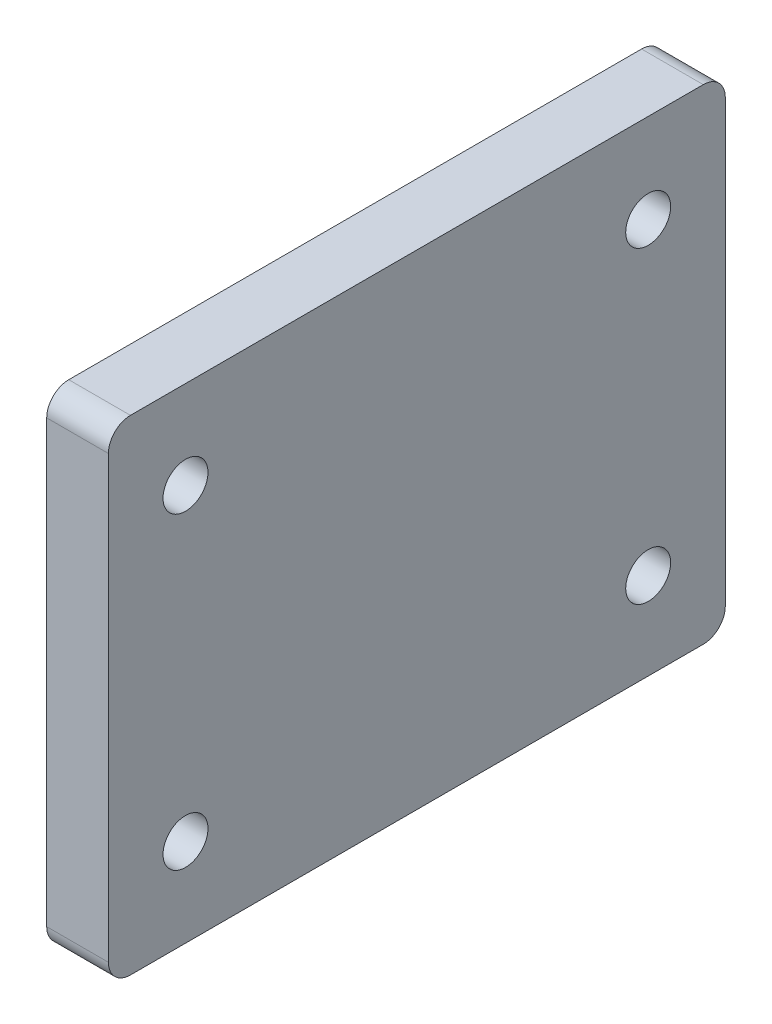
SolidWorks part; units mm, degrees
ref_plane "Front Plane" through (0, 0, 0) normal (0, 0, 1) x (1, 0, 0)
ref_plane "Top Plane" through (0, 0, 0) normal (0, 1, 0) x (1, 0, 0)
ref_plane "Right Plane" through (0, 0, 0) normal (1, 0, 0) x (0, 0, -1)
sketch "Sketch1" plane through (0, 0, 0) normal (1, 0, 0) x (0, 0, -1)
  line L1 (-70, -55) -> (70, -55)
  line L2 (-70, -55) -> (-70, 55)
  line L3 (-70, 55) -> (70, 55)
  line L4 (70, -55) -> (70, 55)
  line L5 (-70, -55) -> (70, 55) construction
  line L6 (-70, 55) -> (70, -55) construction
  point P0 (0, 0)
  dimension "D1" = 140
  dimension "D2" = 110
extrude "Boss-Extrude1" add sketch "Sketch1" along normal blind 14
fillet "Fillet1" radius 5 4 edges at (7, -55, -70) (7, 55, -70) (7, -55, 70) (7, 55, 70)
sketch "Sketch3" plane through (14, 0, 0) normal (1, 0, 0) x (0, 0, -1)
  circle A0 centre (-40, 30) radius 7 construction
  dimension "D1" = 14
sketch "Sketch4" plane through (14, 0, 0) normal (1, 0, 0) x (0, 0, -1)
  circle A0 centre (-40, 30) radius 7 construction
  dimension "D1" = 14
hole_wizard "M12 Tapped Hole1" positions "Sketch5" profile "Sketch6" tap size "M12" standard "GB"
sketch "Sketch5" plane through (0, 0, 0) normal (-1, 0, 0) x (0, 0, 1)
  point P0 (-52.5, 34.7566)
  point P2 (52.4997, 35)
  point P4 (52.5, -35)
  point P6 (-52.5, -35.2434)
  dimension "D1" = 105
  dimension "D2" = 70
  dimension "D3" = 70
  dimension "D4" = 52.5
  dimension "D5" = 35
  dimension "D6" = 105
sketch "Sketch6" plane through (0, 34.7566, -52.5) normal (0, 1, 0) x (0, 0, 1)
  line L0 (0, 0) -> (0, 35.8144)
  line L1 (0, 35.8144) -> (5.1, 32.75)
  line L2 (5.1, 32.75) -> (5.1, 0.925)
  line L3 (5.1, 0.925) -> (6.025, 0)
  line L5 (6.025, 0) -> (0, 0)
  line L6 (-5.1, 0.925) -> (-6.025, 0) construction
  line L10 (0, 35.8144) -> (-5.1, 32.75) construction
  line L11 (0, -6.35) -> (0, 107.95) construction
  dimension "螺纹孔钻头直径" = 10.2
  dimension "螺纹孔钻头深度" = 32.75
  dimension "近端锥形沉头孔直径" = 12.05
  dimension "近端锥形沉头孔角度" = 90
  dimension "导头角度" = 118
cosmetic thread "Cosmetic Thread 1" parameters "D1"=24, "D2"=12
cosmetic thread "Cosmetic Thread 2" parameters "D1"=24, "D2"=12
cosmetic thread "Cosmetic Thread 3" parameters "D1"=24, "D2"=12
cosmetic thread "Cosmetic Thread 4" parameters "D1"=24, "D2"=12
